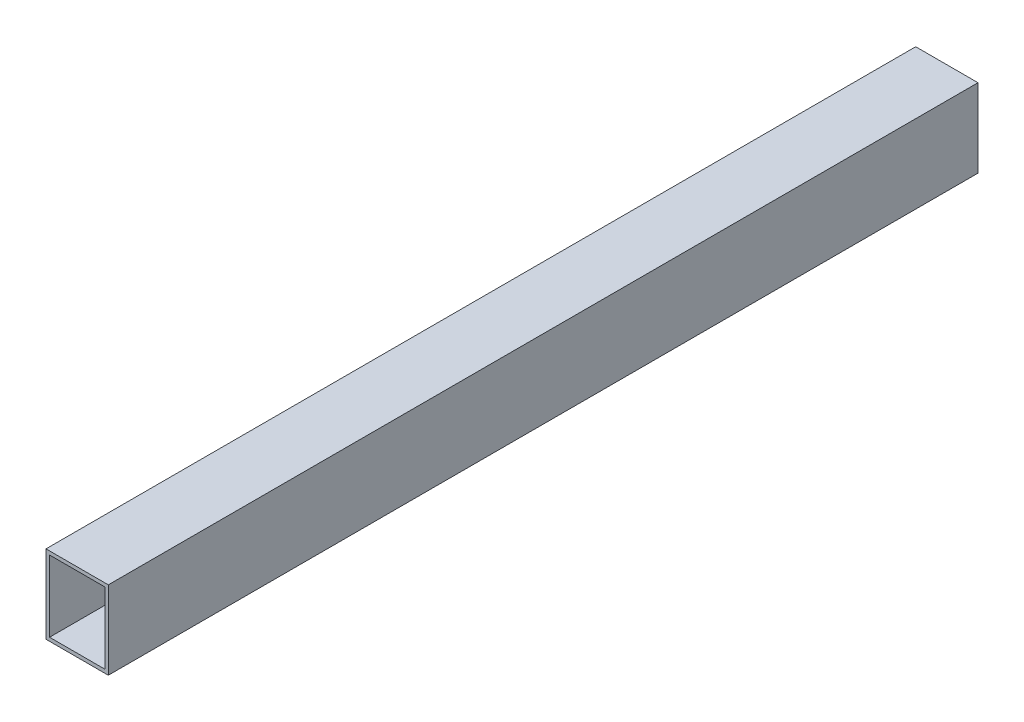
from build123d import *

# Parameters (mm, degrees)
SKETCH1_W           = 35
SKETCH1_H           = 44
SKETCH1_W_2         = 31
SKETCH1_H_2         = 40
BOSS_EXTRUDE1_DEPTH = 488.48935286


with BuildPart() as part:
    # Sketch1 → Boss-Extrude1 (new body)
    with BuildSketch(Plane.XY):
        Rectangle(SKETCH1_W, SKETCH1_H)
        Rectangle(SKETCH1_W_2, SKETCH1_H_2, mode=Mode.SUBTRACT)
    extrude(amount=BOSS_EXTRUDE1_DEPTH)


solid = part.part
